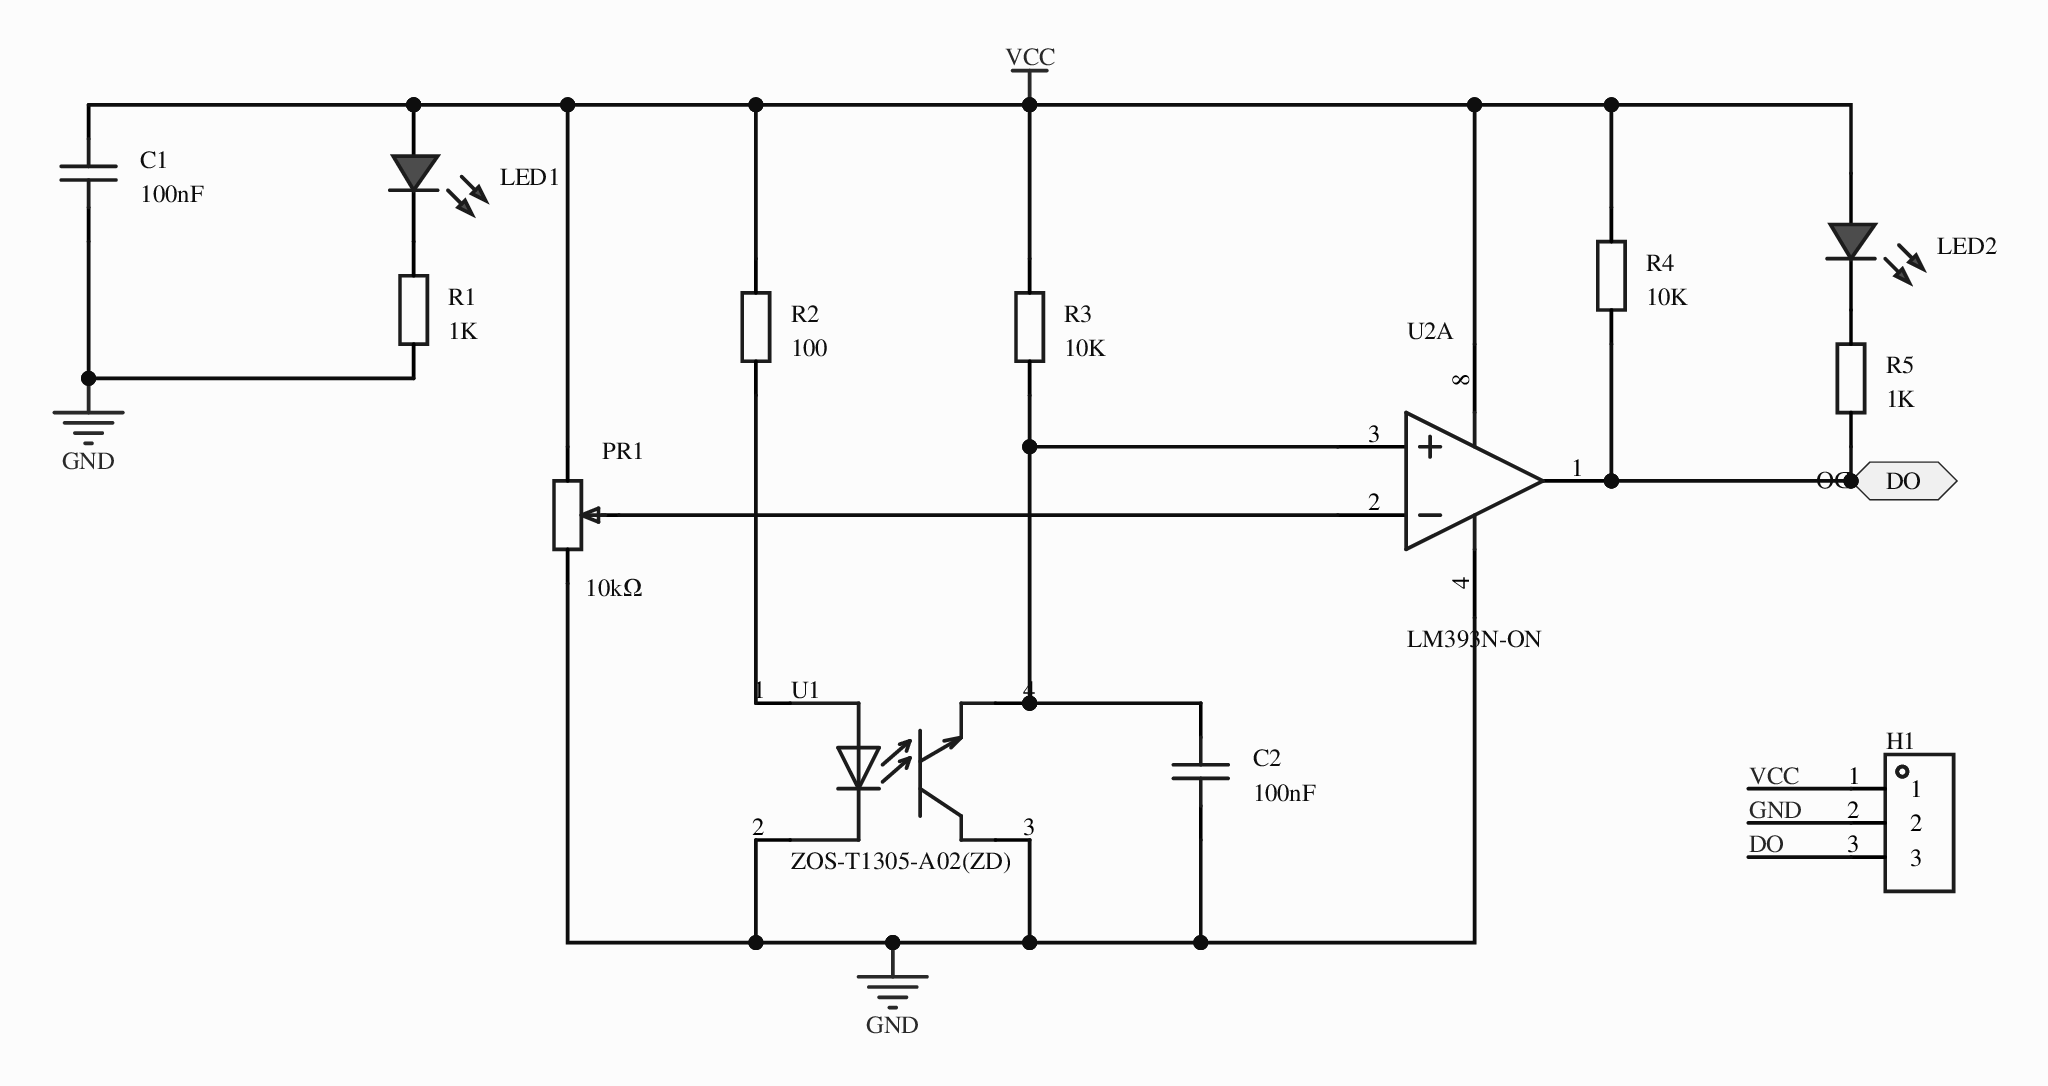
[diagram p0: MISC51709-3.schdoc]
# Altium project MISC51709-2.PrjPcb
1 sheet, 13 parts. Net scope: flat (ports and power ports of the same name join across sheets).
Board file: MISC51709.pcbdoc

## Sheet MISC51709-3.schdoc
size 297 x 209 mm; Version: V1.0; @Project Name: MISC51709; @Update Date: 2026-04-20; @Create Date: 2026-04-20; @Board Name: MISC51709; @Create Time: 16:53:37; @Page Count: 1; @Page No: 1; @Schematic Name: MISC51709; @Update Time: 16:53:37; Size: A4

### Parts
C1  100nF  [C0603]
C2  100nF  [C0603]
H1  (no value)  [HDR-TH_3P-P2.54-V-M]
LED1  (no value)  [LED_TH-3mm]
LED2  (no value)  [LED_TH-3mm]
PR1  10kΩ  [R_3296]
R1  1K  [R0603]
R2  100  [R0603]
R3  10K  [R0603]
R4  10K  [R0603]
R5  1K  [R0603]
U1  ZOS-T1305-A02(ZD)  [OPTO-TH_ZOS-T1305-A02]
U2  LM393N-ON  [PDIP-8_L9.6-W6.4-P2.54-LS7.9-BL]  (part A of 2)

### Ports
DO (bidir)

### Nets
GND: C1.1 C2.1 H1.2 PR1.1 R1.1 U1.2(C) U1.3(COL) U2.4(+VS)
VCC: C1.2 H1.1 LED1.1(C) LED2.1(C) PR1.3 R2.2 R3.2 R4.2 U2.8(-VS)
DO: H1.3 R4.1 R5.1 U2.1(OUTA) ; port DO
NetC2_2: C2.2 R3.1 U1.4(EM) U2.3(INA+)
NetLED1_2: LED1.2(A) R1.2
NetLED2_2: LED2.2(A) R5.2
NetPR1_2: PR1.2 U2.2(INA-)
NetR2_1: R2.1 U1.1(A)

### Library data of the parts
C1 C2 = CAP_0603: Symbol: Capacitance; ConvertToPcb: yes; ModelId: ac125912035d415993ca9572d50418b10819f05c4eef4c71ace90d822a990e87; ModelName: C0603_L1.6-W0.8-H0.8; ModelTransform: 62.992,31.496,0,0,0,0,0,0,0; Device: CAP_0603; AddInBom: yes; Supplier Footprint: 0603; FootprintName: C0603; Value: 100nF
H1 = HDR-M_2.54_1x3P: AddInBom: yes; ModelId: bb473b6d38ff42a99216a4fcdbdcc4cb0819f05c4eef4c71ace90d822a990e87; ModelName: HDR-TH_3P-P2.54-M-LI-1X3P; ModelTransform: 300.03877,100,0,0,0,0,0,0,-118.11; Symbol: HDR-M_2.54_1x3P; Device: HDR-M_2.54_1x3P; ConvertToPcb: yes; FootprintName: HDR-TH_3P-P2.54-V-M; SupplierPart: C2937625; Supplier Footprint: 插件
LED1 LED2 = LED_TH-R_3mm: ConvertToPcb: yes; ModelId: a497c992633541038a38947cdc58012f0819f05c4eef4c71ace90d822a990e87; ModelName: LED-TH-3mm_R; ModelTransform: 141.274,153.327,0,0,0,0,-5.984,0,-137.795; Symbol: LED_TH-R; Device: LED_TH-R_3mm; AddInBom: yes; FootprintName: LED_TH-3mm; Supplier Footprint: 插件
PR1 = R_3296: ConvertToPcb: yes; ModelId: b182808559bb43bda9e7de64b64134cb0819f05c4eef4c71ace90d822a990e87; ModelName: 3296W; ModelTransform: 373.98,188.96,590.49,180,0,0,0,0,-140; Symbol: R_3296; Device: R_3296; AddInBom: yes; Supplier Footprint: 直插; FootprintName: R_3296; Value: 10kΩ
R1-R5 = Res_0603: Symbol: 电阻; ConvertToPcb: yes; ModelId: fc143cca1e79419f9cd78b61e9279f080819f05c4eef4c71ace90d822a990e87; ModelTransform: 31.8897,63.7794,0,90,0,0,0,0,0; Device: Res_0603; AddInBom: yes; Supplier Footprint: 0603; FootprintName: R0603; ModelName: R0603
  R1 R5: Value: 1K
  R2: Value: 100
  R3 R4: Value: 10K
U1 = ZOS-T1305-A02(ZD): 槽宽:5.2mm;暗电流:100nA;峰值波长:940nm;正向压降(Vf):1.2V;; Manufacturer: Chau Light(洲光源); AddInBom: yes; ModelId: 2080340deda04824aea7cea81a5d00dc0819f05c4eef4c71ace90d822a990e87; ModelTransform: 503.936,251.968,0,0,0,0,0,0,-196.85; Slot Width: 5.2mm; Load Voltage: 30V; Output Current: 10mA; Dark Current: 100nA; Peak Wavelength: 940nm; Rise Time: 15us; Voltage - Forward(Vf): 1.2V; Symbol: ZOS-T1305-A02(ZD); Device: ZOS-T1305-A02(ZD); LCSC Part Name: 对射式光电开关; SupplierPart: C457839; ManufacturerPart: ZOS-T1305-A02(ZD); Supplier Footprint: DIP-4; JLCPCB Part Class: Extended Part; Datasheet: https://item.szlcsc.com/datasheet/ZOS-T1305-A02(ZD)/461458.html; Supplier: LCSC; ConvertToPcb: yes; FootprintName: OPTO-TH_ZOS-T1305-A02; ModelName: OPTO-TH_ZOS-T1305-A02; Fall Time: 15us; Length: 12.8mm; Width: 6.4mm; Height: 6.9mm; Operating Temperature: -25℃~+85℃
U2 = LM393N-ON: 输入失调电压(Vos):5mV;输入偏置电流(Ib):250nA;; Manufacturer: onsemi(安森美); Relevance: []; AddInBom: yes; ModelId: dc5e4f88791a4763b9523ab1244c0ba10819f05c4eef4c71ace90d822a990e87; ModelTransform: 377.952,309.842,0,0,0,0,0,0,-110.236; Input Offset Voltage (Vos): 5mV; Input Bias Current (Ib): 250nA; Supply Voltage: 1V~18V；2V~36V; Output Type: 开集; Symbol: LM393N-ON; Device: LM393N-ON; LCSC Part Name: LM393N-ON; SupplierPart: C3658682; ManufacturerPart: LM393N-ON; Supplier Footprint: PDIP-8; JLCPCB Part Class: Extended Part; Datasheet: https://atta.szlcsc.com/upload/public/pdf/source/20230915/E90C6EDC3B9A547638D85557898CF661.pdf; Supplier: LCSC; ConvertToPcb: yes; FootprintName: PDIP-8_L9.6-W6.4-P2.54-LS7.9-BL; ModelName: PDIP-8_L9.6-W6.4-P2.54-LS7.9-BL; Input Hysteresis Voltage (Vhys): -; Common Mode Rejection Ratio (CMRR): -; Output Mode: -; Operating Temperature: 0℃~+70℃